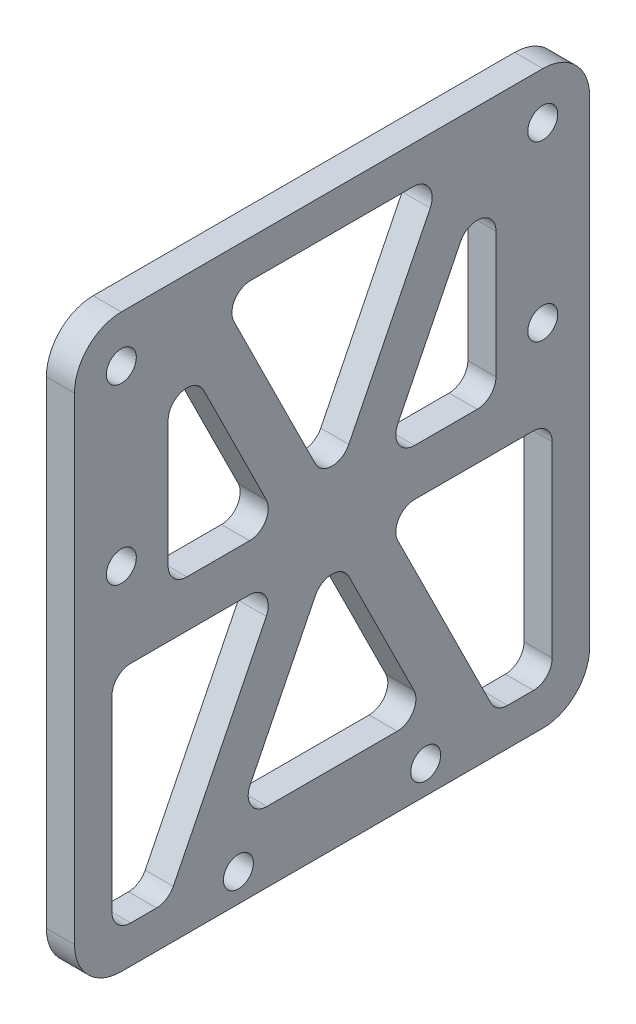
from build123d import *

# Parameters (mm, degrees)
SKETCH_2_W          = 55
SKETCH_2_H          = 61
EXTRUDE_1_DEPTH     = 3
SKETCH_3_R          = 1.6
CUT_EXTRUDE_1_DEPTH = 3
FILLET_1_R          = 5
CUT_EXTRUDE_2_DEPTH = 3
FILLET_2_R          = 2


with BuildPart() as part:
    # 草图2 → 凸台-拉伸1 (new body)
    with BuildSketch(Plane(origin=(0, 0, 0), x_dir=(0, 0, -1), z_dir=(1, 0, 0))):
        with Locations((27.5, 30.5)):
            Rectangle(SKETCH_2_W, SKETCH_2_H)
    extrude(amount=EXTRUDE_1_DEPTH)

    # 草图3 → 切除-拉伸1 (cut)
    with BuildSketch(Plane.ZY):
        with Locations((-5, 56)):
            Circle(SKETCH_3_R)
        with Locations((-5, 37.5)):
            Circle(SKETCH_3_R)
        with Locations((-50, 56)):
            Circle(SKETCH_3_R)
        with Locations((-50, 37.5)):
            Circle(SKETCH_3_R)
        with Locations((-37.5, 3)):
            Circle(SKETCH_3_R)
        with Locations((-17.5, 3)):
            Circle(SKETCH_3_R)
    extrude(amount=-CUT_EXTRUDE_1_DEPTH, mode=Mode.SUBTRACT)

    # 圆角1
    fillet_1_edges = [part.edges().sort_by_distance(p)[0] for p in [
        (1.5, 61, 0),
        (1.5, 61, -55),
        (1.5, 0, -55),
        (1.5, 0, 0),
    ]]
    fillet(fillet_1_edges, radius=FILLET_1_R)

    # 草图4 → 切除-拉伸2 (cut)
    with BuildSketch(Plane.ZY):
        Polygon((-39.417495765, 57), (-27.5, 33), (-15.582504235, 57), align=None)
        Polygon((-45, 57), (-45, 33), (-33.082504235, 33), align=None)
        Polygon((-21.917495765, 33), (-10, 57), (-10, 33), align=None)
        Polygon((-10, 28), (-21.917495765, 28), (-10, 4), (-4, 4), (-4, 28), align=None)
        Polygon((-37.679527633, 7.5), (-27.5, 28), (-17.320472367, 7.5), align=None)
        Polygon((-45, 28), (-33.082504235, 28), (-45, 4), (-51, 4), (-51, 28), align=None)
    extrude(amount=-CUT_EXTRUDE_2_DEPTH, mode=Mode.SUBTRACT)

    # 圆角2
    fillet_2_edges = [part.edges().sort_by_distance(p)[0] for p in [
        (1.5, 57, -45),
        (1.5, 33, -33.082504235),
        (1.5, 33, -45),
        (1.5, 57, -39.417495765),
        (1.5, 57, -15.582504235),
        (1.5, 33, -27.5),
        (1.5, 28, -27.5),
        (1.5, 7.5, -17.320472367),
        (1.5, 7.5, -37.679527633),
        (1.5, 28, -4),
        (1.5, 4, -4),
        (1.5, 4, -10),
        (1.5, 28, -21.917495765),
        (1.5, 4, -51),
        (1.5, 28, -51),
        (1.5, 28, -33.082504235),
        (1.5, 4, -45),
        (1.5, 33, -10),
        (1.5, 33, -21.917495765),
        (1.5, 57, -10),
    ]]
    fillet(fillet_2_edges, radius=FILLET_2_R)


solid = part.part
